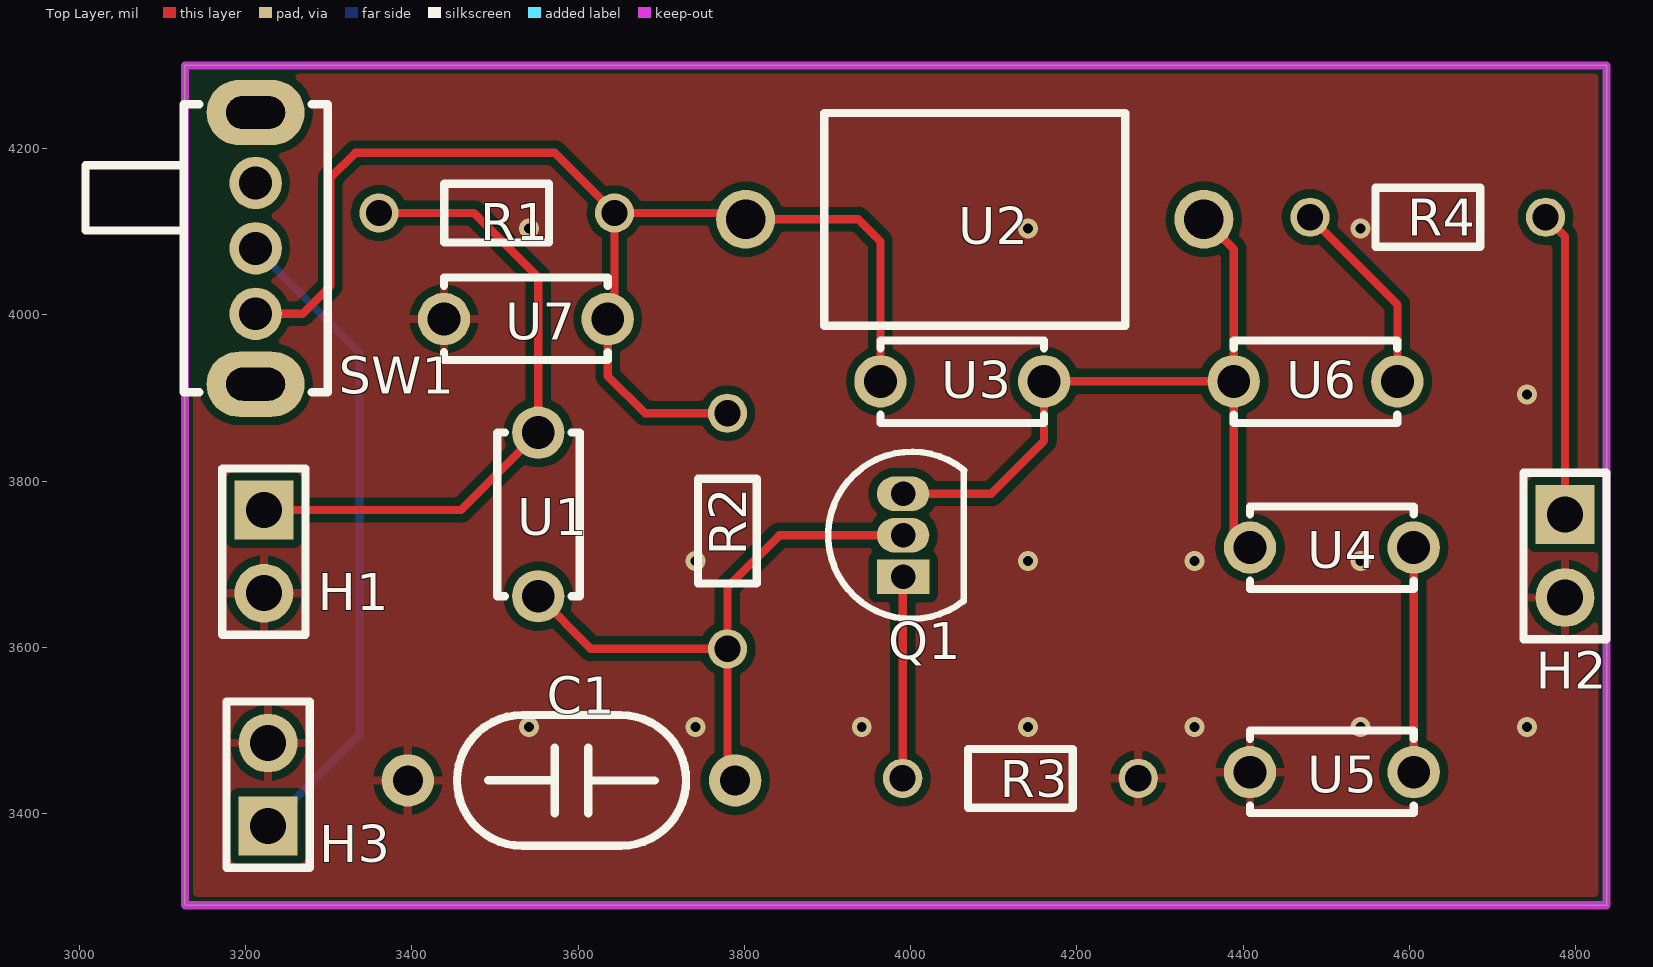
[diagram p0: Top Layer view]
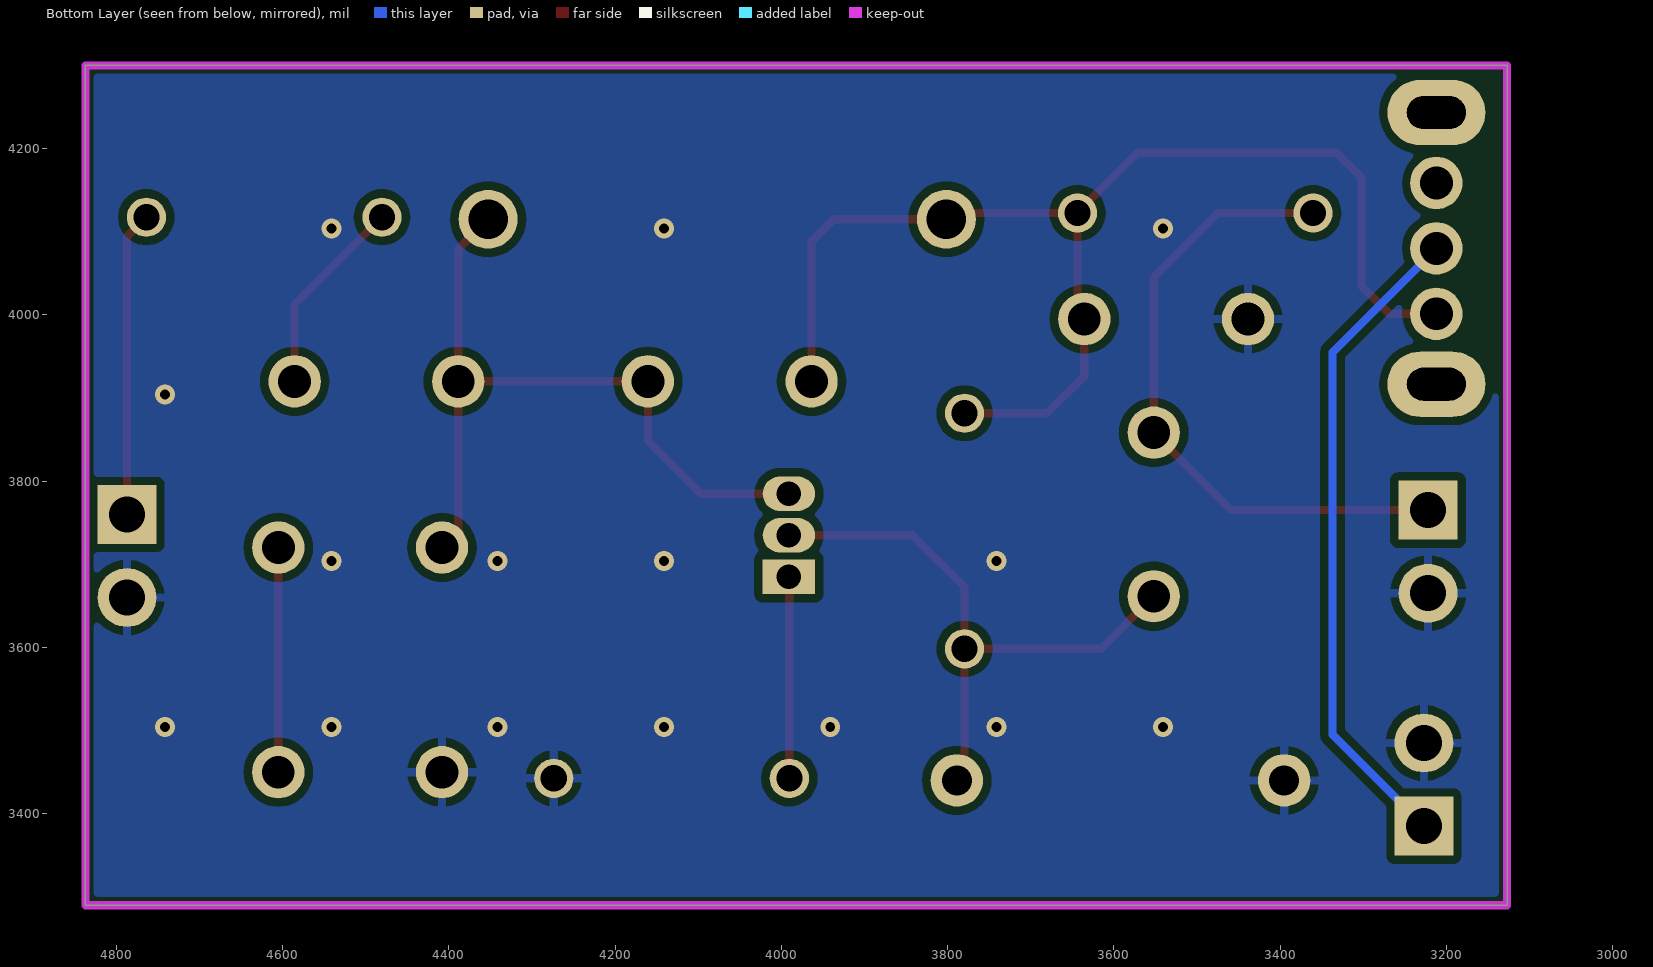
[diagram p1: Bottom Layer view, seen from below]
# Altium PCB MISC51145.pcbdoc
Units mil, origin at the board's own origin, x right, y up, seen from the top; angles counter-clockwise.
Board outline 1710 x 1010 mil, 2 copper layers (Top Layer, Bottom Layer), stack 62.206 mil thick; 17 components, 10 nets, 38 pads, 15 vias.

## Layer stack, top to bottom
Top Solder Mask Layer: solder mask 0.394, Dk 3.3
Top Layer: signal copper 1.379
Dielectric1: surface 59.449, FR4, Dk 4.5
Bottom Layer: signal copper 1.378
Bottom Solder Mask Layer: solder mask 0.394, Dk 3.3

## Board outline
3127.1,4300 3127.1,3290 4837.1,3290 4837.1,4300

## Design rules (kind name [scope] priority, off if disabled: settings)
BoardOutlineClearance copperThickness2oz_1 [All] p2 off: genericclearance=7.99 ignorepadtopadclearanceinfootprint=FALSE except(0: Arc-SplitContinuation Track-SplitContinuation SMDPad-SplitContinuation THPad-SplitContinuation Via-SplitContinuation Fill-SplitContinuation Region-SplitContinuation Poly-SplitContinuation Text-SplitContinuation Hole-SplitContinuation; 5.98: Arc-CutoutEdge SMDPad-CutoutEdge THPad-CutoutEdge Via-CutoutEdge Fill-CutoutEdge Region-CutoutEdge Text-CutoutEdge; 6.93: Hole-OutlineEdge Hole-CutoutEdge; 10: Poly-OutlineEdge Poly-CutoutEdge; 11.81: Arc-OutlineEdge Track-OutlineEdge SMDPad-OutlineEdge THPad-OutlineEdge Via-OutlineEdge Fill-OutlineEdge Region-OutlineEdge Text-OutlineEdge Track-CutoutEdge)
BoardOutlineClearance copperThickness1oz_1 [All] p4: genericclearance=4.02 ignorepadtopadclearanceinfootprint=FALSE except(0: Arc-SplitContinuation Track-SplitContinuation SMDPad-SplitContinuation THPad-SplitContinuation Via-SplitContinuation Fill-SplitContinuation Region-SplitContinuation Poly-SplitContinuation Text-SplitContinuation Hole-SplitContinuation; 6: SMDPad-CutoutEdge THPad-CutoutEdge Via-CutoutEdge Fill-CutoutEdge Region-CutoutEdge Text-CutoutEdge; 6.93: Hole-OutlineEdge Hole-CutoutEdge; 10: Poly-OutlineEdge Poly-CutoutEdge; 11.8: Arc-OutlineEdge Track-OutlineEdge SMDPad-OutlineEdge THPad-OutlineEdge Via-OutlineEdge Fill-OutlineEdge Region-OutlineEdge Text-OutlineEdge; 11.81: Arc-CutoutEdge Track-CutoutEdge)
Clearance copperThickness2oz [All] p1 off: gap=7.99 ignorepadtopadclearanceinfootprint=FALSE except(5.98: SMDPad-Track SMDPad-SMDPad THPad-Track SMDPad-THPad THPad-THPad Track-Via SMDPad-Via THPad-Via Via-Via Fill-Track Region-Track Fill-SMDPad Region-SMDPad Fill-THPad Region-THPad Fill-Via Region-Via Fill-Fill Fill-Region Region-Region Arc-Track Arc-SMDPad Arc-THPad Arc-Via Fill-Arc Region-Arc Arc-Arc Text-Track SMDPad-Text Text-THPad Text-Via Fill-Text Region-Text Arc-Text Text-Text; 6.93: Hole-Track Hole-SMDPad Hole-THPad Hole-Via Fill-Hole Region-Hole Hole-Arc Hole-Text; 10: Poly-Track Poly-SMDPad Poly-THPad Poly-Via Poly-Fill Poly-Region Poly-Poly Poly-Arc Poly-Text Poly-Hole)
Clearance copperThickness1oz [All] p3: gap=4.02 ignorepadtopadclearanceinfootprint=FALSE except(5.98: SMDPad-Track SMDPad-SMDPad THPad-Track SMDPad-THPad THPad-THPad Track-Via SMDPad-Via THPad-Via Via-Via Fill-Track Region-Track Fill-SMDPad Region-SMDPad Fill-THPad Region-THPad Fill-Via Region-Via Fill-Fill Fill-Region Region-Region; 6: Arc-Track Arc-SMDPad Arc-THPad Arc-Via Fill-Arc Region-Arc Arc-Arc Text-Track SMDPad-Text Text-THPad Text-Via Fill-Text Region-Text Arc-Text Text-Text; 6.93: Hole-Track Hole-SMDPad Hole-THPad Hole-Via Fill-Hole Region-Hole Hole-Arc Hole-Text; 10: Poly-Track Poly-SMDPad Poly-THPad Poly-Via Poly-Fill Poly-Region Poly-Poly Poly-Arc Poly-Text Poly-Hole)
DiffPairsRouting differentialPair [All] p1: maxlimit=6 minlimit=6 mostfreqgap=6 toplayer_minwidth=5 toplayer_prefwidth=10 toplayer_maxwidth=100 toplayer_mingap=6 toplayer_prefgap=6 toplayer_maxgap=6 bottomlayer_minwidth=5 bottomlayer_prefwidth=10 bottomlayer_maxwidth=100 bottomlayer_mingap=6 bottomlayer_prefgap=6 bottomlayer_maxgap=6 maxuncoupledlength=10
HoleToHoleClearance otherClearance [All] p1: gap=11.81 allowstackedmicrovias=TRUE
Length netLength [All] p1: minlimit=0 maxlimit=0
MatchedLengths netLengthTolerance [All] p1: tolerance=1000
PasteMaskExpansion pasteMaskExpansion [All] p1: expansion=0
PlaneConnect innerPlane [All] p1: planeconnectstyle=Relief reliefexpansion=20 reliefentries=4 reliefconductorwidth=10 reliefairgap=10
PolygonConnect copperRegion [(InNet('GND'))] p1: connectstyle=Relief reliefconductorwidth=10 reliefentries=4 polygonreliefangle="90 Angle" airgapwidth=10 via.connectstyle=Relief via.reliefconductorwidth=10 via.reliefentries=4 via.polygonreliefangle="90 Angle" via.airgapwidth=10
RoutingVias viaSize [All] p1: holewidth=12.01 width=24.02 viastyle="Through Hole" minholewidth=11.81 minwidth=19.68 maxholewidth=248.03 maxwidth=393.7
SolderMaskExpansion solderMaskExpansion [IsVia] p1: expansion=-1000 istentingtop=TRUE
SolderMaskExpansion solderMaskExpansion [All] p2: expansion=2 istentingtop=FALSE
Width copperThickness2oz_2 [All] p1 off: maxlimit=100 minlimit=8 preferedwidth=10
Width copperThickness1oz_2 [All] p2: maxlimit=100 minlimit=5 preferedwidth=10

## Components (designator, comment, footprint, x,y, rotation, side; value= is the part's Value field where it differs from the comment)
C1 "1nF" CAP-TH_L7.0-W4.0-P10.00-D0.6-1 3592.1,3440 r0 top
H1 "" HDR-TH_2P-P2.54-V-M-1 3222.1,3715.2 r270 top
H2 "" HDR-TH_2P-P2.54-V-M-1 4787.1,3710 r270 top
H3 "" HDR-TH_2P-P2.54-V-M-1 3227.1,3435 r90 top
Q1 "2N2222A" TO-92-3_L5.1-W4.1-P1.27-L-1 3990.97,3734.89 r90 top
R1 "2.2kΩ" Res_1/8W 3502.1,4120 r0 top
R2 "20kΩ" Res_1/8W 3782.1,3740 r90 top
R3 "220Ω" Res_1/8W 4132.1,3445 r180 top
R4 "50Ω" Res_1/8W 4622.1,4115 r0 top
SW1 "" 拨动开关_侧 3212.1,4080 r270 top
U1 "100nF" CAP-TH_L5.0-W2.5-P5.00-D1.0 3552.1,3760 r90 top
U2 "0.08uH" IND-TH_BD6.5-W9.2-LS14.0-D0.8 4077.1,4115 r0 top
U3 "25pF" CAP-TH_L5.0-W2.5-P5.00-D1.0 4062.1,3920 r0 top
U4 "10pF" CAP-TH_L5.0-W2.5-P5.00-D1.0 4506.6,3720.2 r0 top
U5 "30pF" CAP-TH_L5.0-W2.5-P5.00-D1.0 4506.6,3449.96 r180 top
U6 "10pF" CAP-TH_L5.0-W2.5-P5.00-D1.0 4487.1,3920 r0 top
U7 "100nF" CAP-TH_L5.0-W2.5-P5.00-D1.0 3537.1,3995 r180 top

## Footprints (in the part's own frame and the unit in brackets; to place one, negate y for a bottom-side part, rotate by r counter-clockwise, add the part's x,y. Pads: shape width x height; smd on the part's side, far side on the other; paste and mask are expansions set on the pad)
CAP-TH_L5.0-W2.5-P5.00-D1.0 [mm]
  round 1.6 hole 1: 1(-2.5,0) 2(2.5,0)
  silkscreen extent -2.5,-1.27 2.5,1.25
CAP-TH_L7.0-W4.0-P10.00-D0.6-1 [mm]
  round 1.6 hole 0.914 paste+0 mask+0.05: 1(-5,0) 2(5,0)
  silkscreen extent -3.5,-2 3.5,2
HDR-TH_2P-P2.54-V-M-1 [mm]
  rect 1.8x1.8 hole 1.1: 1(-1.27,0)
  round 1.8 hole 1.1: 2(1.27,0)
  silkscreen extent -2.54,-1.27 2.54,1.27
IND-TH_BD6.5-W9.2-LS14.0-D0.8 [mm]
  round 1.8 hole 1.2 paste+0 mask+0.05: 1(-7,0) 2(7,0)
  silkscreen extent -4.6,-3.25 4.6,3.25
Res_1/8W [mil]
  round 47.2 hole 31.5 paste+0 mask+2: 1(-141.7,2.48) 2(141.7,2.48)
  silkscreen extent -63,-33 63,38
TO-92-3_L5.1-W4.1-P1.27-L-1 [mm]
  rect 1.05x1.6 hole 0.75: 1(-1.27,0)
  oval 1.05x1.6 hole 0.75: 2(0,0) 3(1.27,0)
  silkscreen extent -2.55,-1.87 2.55,2.29
拨动开关_侧 [mil]
  round 63 hole 39.4 paste+0 mask+2: 1(-78.7,0) 2(0,0) 3(78.7,0)
  oval 78.7x118.1 hole 39.4 slot 70.9 at 90 deg paste+0 mask+2: 4(163.4,0) 5(-163.4,0)
  silkscreen extent -173,-205 173,87

## Via types
v1: diameter 24.02, hole 12, Top Layer to Bottom Layer, 15 vias

## Nets (pads, with @x,y where several pads share a name; then routed paths per layer and width w, separated by ;. In a path a pad name is that pad's centre, name@x,y a point inside that pad or via, vN(x,y) a via of type N, cw(c..) or ccw(c..) an arc to the next point about the centre after c; other vN are vias at no path point)
$1N1: H1.1 R1.1 U1.2 | length 779
  Top Layer w10: H1.1 3458.88,3765.2 U1.2 3552.1,4045 3474.62,4122.48 R1.1
$1N3: C1.2 Q1.2 R2.1 U1.1 | length 727.3
  Top Layer w10: U1.1 3615.38,3598.3 R2.1 ; C1.2 3779.62,3449.33 R2.1 ; Q1.2 3841.99,3734.89 3779.62,3672.52 R2.1
$1N5: Q1.1 R3.2 | length 242.6
  Top Layer w10: R3.2 3990.4,3684.32 Q1.1
$1N6: Q1.3 U2.2 U3.2 U4.1 U6.1 | length 913.4
  Top Layer w10: Q1.3 4096.99,3784.89 4160.52,3848.43 U3.2 U6.1 ; U2.2 4388.68,4079.01 U6.1 ; U4.1 4388.68,3739.7 U6.1
$1N8: U4.2 U5.1 | length 270.2
  Top Layer w10: U5.1 U4.2
$1N9: R4.1 U6.2 | length 241
  Top Layer w10: R4.1 4585.52,4012.35 U6.2
$1N10: H2.1 R4.2 | length 367.1
  Top Layer w10: R4.2 4787.1,4094.18 H2.1
$1N13: R1.2 R2.2 SW1.3 U2.1 U3.1 U7.1 | length 1483
  Top Layer w10: SW1.3 3268.4,4001.3 3302.1,4035 3302.1,4165 3332.1,4195 3572.1,4195 3643.8,4123.3 R1.2 ; R2.2 3680.4,3881.7 3635.53,3926.57 U7.1 3643.8,4003.28 R1.2 ; U3.1 3963.68,4088.43 3937.1,4115 U2.1 3794.03,4122.48 R1.2
$1N14: H3.1 SW1.2 | length 792.3
  Bottom Layer w10: SW1.2 3337.1,3955 3337.1,3495 H3.1
GND: C1.1 H1.2 H2.2 H3.2 R3.1 U5.2 U7.2
  other v1: 3541.2,3504.1 3741.2,3504.1 3941.2,3504.1 4141.2,3504.1 4341.2,3504.1 4541.2,3504.1 4741.2,3504.1 3741.2,3704.1 4141.2,3704.1 4341.2,3704.1 4541.2,3704.1 4741.2,3904.1 3541.2,4104.1 4141.2,4104.1 4541.2,4104.1
pads on no net: SW1.1 SW1.4 SW1.5

## Polygon pours and split planes (outlines as drawn)
GND on Top Layer (solid, remove dead copper, pour order 0): 3007.1,4460 3007.1,3000 5217.1,3000 5217.1,4460
GND on Bottom Layer (solid, remove dead copper, pour order 2): 3067.1,4360 3067.1,3155 4937.1,3155 4937.1,4360

## Keep-outs
Board Outline Layer:
  the board outline again, w10